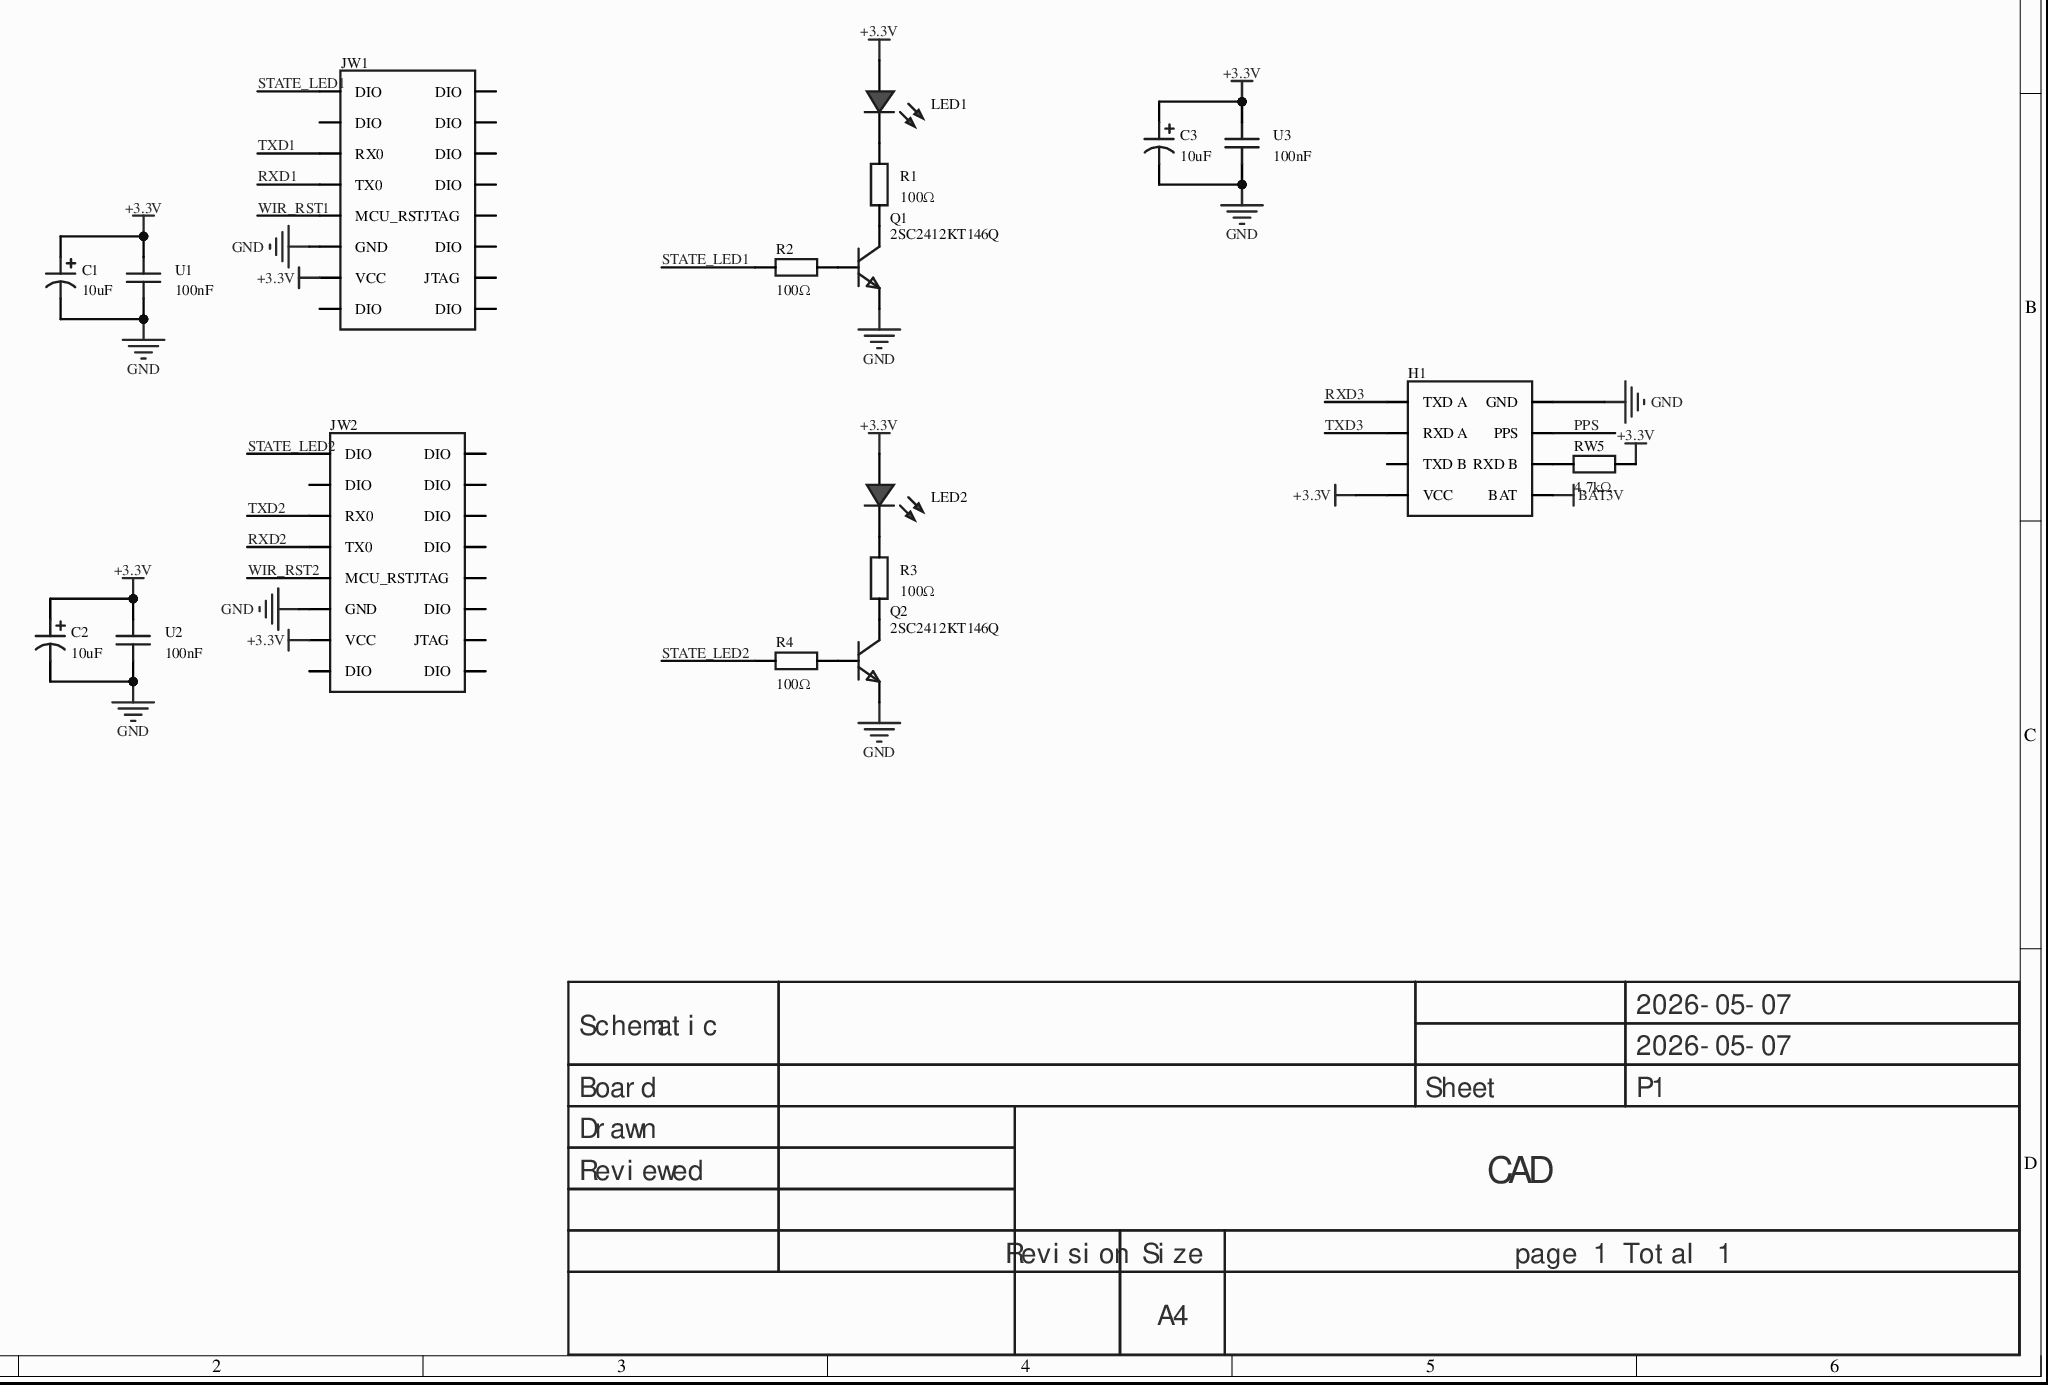
[diagram p0: MISC49947-3.schdoc]
# Altium project MISC49947-2.PrjPcb
1 sheet, 18 parts. Net scope: global (net labels, ports and power ports of the same name join across sheets).
Board file: MISC49947.pcbdoc

## Sheet MISC49947-3.schdoc
size 297 x 209 mm; Version: V1.0; @Project Name: MISC49947; @Update Date: 2026-05-07; @Create Date: 2026-05-07; @Board Name: MISC49947; @Create Time: 10:01:02; @Page Count: 1; @Page No: 1; @Schematic Name: MISC49947; @Update Time: 10:01:02; Size: A4

### Parts
C1  10uF  [CAP-TH_BD5.0-P2.00-D0.8-FD-10UF50VC110GL]
C2  10uF  [CAP-TH_BD5.0-P2.00-D0.8-FD-10UF50VC110GL]
C3  10uF  [CAP-TH_BD5.0-P2.00-D0.8-FD-10UF50VC110GL]
H1  (no value)  [HDR-TH_8P-P2.54-V-F-R2-C4-S2.54-1]
JW1  (no value)  [HDR-TH_16P-P2.54-V-F-R2-C8-S2.54-1]
JW2  (no value)  [HDR-TH_16P-P2.54-V-F-R2-C8-S2.54-1]
LED1  (no value)  [LED_TH-3mm]
LED2  (no value)  [LED_TH-3mm]
Q1  2SC2412KT146Q  [SOT-346_L2.9-W1.6-P1.90-LS2.8-TR-CW-1]
Q2  2SC2412KT146Q  [SOT-346_L2.9-W1.6-P1.90-LS2.8-TR-CW-1]
R1  100Ω  [Res_1/8W]
R2  100Ω  [Res_1/8W]
R3  100Ω  [Res_1/8W]
R4  100Ω  [Res_1/8W]
RW5  4.7kΩ  [Res_1/8W]
U1  100nF  [CAP-TH_L5.0-W2.5-P5.00-D1.0]
U2  100nF  [CAP-TH_L5.0-W2.5-P5.00-D1.0]
U3  100nF  [CAP-TH_L5.0-W2.5-P5.00-D1.0]

### Nets
+3.3V: C1.1 C2.1 C3.1 H1.7(VCC) JW1.13(VCC) JW2.13(VCC) LED1.1(C) LED2.1(C) RW5.2 U1.1 U2.1 U3.1
BAT3V: H1.8(BAT)
GND: C1.2 C2.2 C3.2 H1.2(GND) JW1.11(GND) JW2.11(GND) Q1.1(E) Q2.1(E) U1.2 U2.2 U3.2
PPS: H1.4(PPS)
RXD1: JW1.7(TX0)
RXD2: JW2.7(TX0)
RXD3: H1.1(TXD_A)
STATE_LED1: JW1.1(DIO) R2.2
STATE_LED2: JW2.1(DIO) R4.2
TXD1: JW1.5(RX0)
TXD2: JW2.5(RX0)
TXD3: H1.3(RXD_A)
WIR_RST1: JW1.9(MCU_RST)
WIR_RST2: JW2.9(MCU_RST)
NetH1_6: H1.6(RXD_B) RW5.1
NetLED1_2: LED1.2(A) R1.2
NetLED2_2: LED2.2(A) R3.2
NetQ1_2: Q1.2(B) R2.1
NetQ1_3: Q1.3(C) R1.1
NetQ2_2: Q2.2(B) R4.1
NetQ2_3: Q2.3(C) R3.1

Not connected (* = marked no-connect by the designer): H1 5(TXD_B); JW1 2(DIO) 3(DIO) 4(DIO) 6(DIO) 8(DIO) 10(JTAG) 12(DIO) 14(JTAG) 15(DIO) 16(DIO); JW2 2(DIO) 3(DIO) 4(DIO) 6(DIO) 8(DIO) 10(JTAG) 12(DIO) 14(JTAG) 15(DIO) 16(DIO)

### Notes on the sheet
- 2026-05-07
- Schematic
- Board
- Sheet
- P1
- Drawn
- Reviewed
- CAD
- Revision
- Size
- A4
- page 1 Total 1

### Library data of the parts
C1-C3 = 10UF50VC110GL: component 10UF50VC110GL componentdescrip capacitance:10uF; tolerance:±20%; rated voltage:50V; ripple current:120mA@100KHz; equivalent series resistance(ESR):1.6Ω;; Manufacturer: Econd(米朗电子); Tolerance: ±20%; Voltage Rating: 50V; Equivalent Series Resistance(ESR): 1.6Ω; Pin Spacing: 2mm; Lifetime: 5000hrs@105℃; AddInBom: yes; Symbol: 10UF50VC110GL; Device: 10UF50VC110GL; LCSC Part Name: 10uF ±20% 50V; Supplier Part: C46867109; Manufacturer Part: 10UF50VC110GL; Supplier Footprint: 插件,D5xL11mm; JLCPCB Part Class: Extended Part; Datasheet: https://example.com/datasheet/10UF50VC110GL/49031974.html; Supplier: LCSC; Value: 10uF; Ripple Current: 120mA@100KHz; Diameter: 5mm; Height - Seated (Max): 11mm; Operating Temperature: -40℃~+105℃; ConvertToPcb: yes; FootprintName: CAP-TH_BD5.0-P2.00-D0.8-FD-10UF50VC110GL
H1 = HDR-F_2.54_2x4: Symbol: HDR-F-2.54_2x4_1; 3D Model: 64729f32a5874cf59655d275a66f10500819f05c4eef4c71ace90d822a990e87; 3D Model Transform: 399.999,200,0,0,0,0,0,0,-118.11; ConvertToPcb: yes; ModelName: HDR2.54-F-LI-2X4P; Device: HDR-F_2.54_2x4; Supplier Part: C92271; Supplier Footprint: 插件; AddInBom: yes; FootprintName: HDR-TH_8P-P2.54-V-F-R2-C4-S2.54-1
JW1 JW2 = HDR-F_2.54_2x8: Symbol: HDR-F-2.54_2x8_1; 3D Model: f6b5f7d40ec74b809fbaeebc5002f6e00819f05c4eef4c71ace90d822a990e87; 3D Model Transform: 799.99844,200,0,0,0,0,0,0,-118.11; ConvertToPcb: yes; ModelName: HDR2.54-F-LI-2X8P; Device: HDR-F_2.54_2x8; Supplier Part: C30734; Supplier Footprint: 插件; AddInBom: yes; FootprintName: HDR-TH_16P-P2.54-V-F-R2-C8-S2.54-1
LED1 LED2 = LED_TH-R_3mm: ConvertToPcb: yes; ModelId: a497c992633541038a38947cdc58012f0819f05c4eef4c71ace90d822a990e87; ModelName: LED-TH-3mm_R; ModelTransform: 141.274,153.327,0,0,0,0,-5.984,0,-137.795; Symbol: LED_TH-R; Device: LED_TH-R_3mm; AddInBom: yes; FootprintName: LED_TH-3mm; Supplier Footprint: 插件
Q1 Q2 = 2SC2412KT146Q: component 2SC2412KT146Q componentdescrip transistor type:NPN; collector current(Ic):150mA; collector-emitter breakdown voltage(Vceo):50V; power dissipation(Pd):200mW; DC current gain(hFE):120@1mA,6V;; Manufacturer: ROHM(罗姆); 3D Model: a4a06993f12d4e549f90dd43379ebd720819f05c4eef4c71ace90d822a990e87; 3D Model Transform: 110.236,110.49517,0,0,0,0,0,0,0; type: NPN; Current - Collector(Ic): 150mA; Collector - Emitter Voltage VCEO: 50V; Pd - Power Dissipation: 200mW; Transition frequency(fT): 180MHz; Current - Collector Cutoff: 100nA; Vce Saturation(VCE(sat)): 400mV; AddInBom: yes; Symbol: 2SC2412KT146Q; Device: 2SC2412KT146Q; LCSC Part Name: hfe=120~270 NPN 电流:150mA 电压:50V; Supplier Part: C79979; Manufacturer Part: 2SC2412KT146Q; Supplier Footprint: SOT-346; JLCPCB Part Class: Extended Part; Datasheet: https://example.com/datasheet/2SC2412KT146Q/81124.html; Supplier: LCSC; DC Current Gain: 120@1mA,6V; Operating Temperature: -55℃~+150℃; ConvertToPcb: yes; FootprintName: SOT-346_L2.9-W1.6-P1.90-LS2.8-TR-CW-1; ModelName: SOT-346_L2.9-W1.6-P1.90-LS2.8-TR-CW-1
R1-R4 RW5 = Res_AXIAL-1/8W: Symbol: Resistor; 3D Model: b2b5ae7ae4c642178fe0039925c86a3f0819f05c4eef4c71ace90d822a990e87; 3D Model Transform: 282.86,66.88,253.09,0,0,0,0,0,-191; ConvertToPcb: yes; ModelName: RES-TH_BD1.8-L3.2-P7.20-D0.4; Device: Res_AXIAL-1/8W; Supplier Footprint: 轴向引线; AddInBom: yes; FootprintName: Res_1/8W
  R1-R4: Value: 100Ω
  RW5: Value: 4.7kΩ
U1-U3 = 100nF: Symbol: 100NF_C9900015256; 3D Model: 08e3d7481fc7486bb1b263873f51e1e10819f05c4eef4c71ace90d822a990e87; 3D Model Transform: 224.652,98.425,0,0,0,0,-0.005,0,-137.795; AddInBom: yes; ModelName: CAP-TH_BD5.0-W2.5-P5.08; Device: 100nF; LCSC Part Name: 100nF; Supplier Part: C9900015256; Manufacturer Part: 100nF; Supplier Footprint: CAP-TH_L5.0-W2.5-P5.00-D1.0; JLCPCB Part Class: Extended Part; Supplier: LCSC; ConvertToPcb: yes; FootprintName: CAP-TH_L5.0-W2.5-P5.00-D1.0